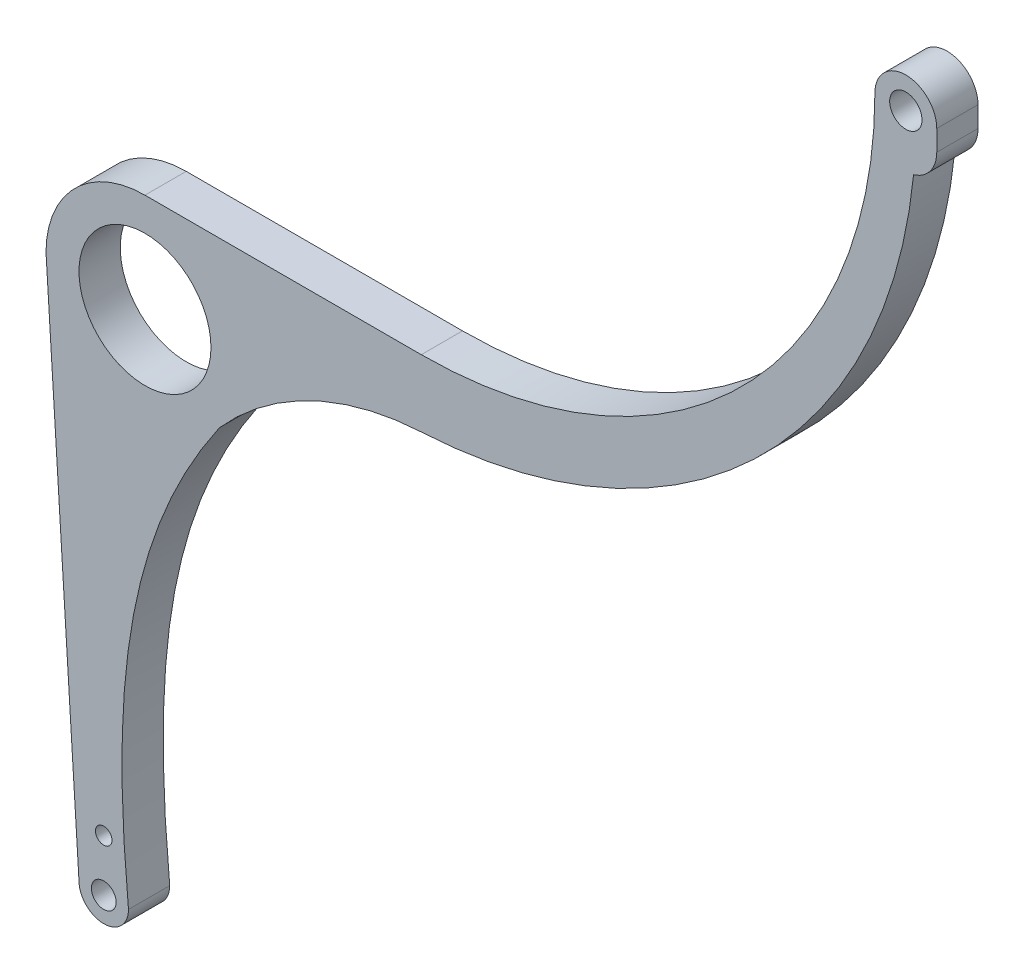
from build123d import *

# Parameters (mm, degrees)
SKETCH_1_R      = 3
SKETCH_1_R_2    = 16
SKETCH_1_R_3    = 3.91899873
SKETCH_1_R_4    = 2
EXTRUDE_1_DEPTH = 10


with BuildPart() as part:
    # 草图1 → 凸台-拉伸1 (new body)
    with BuildSketch(Plane.XY):
        with BuildLine():
            Line((-14, 128), (-6, 0))
            ThreePointArc((-6, 0), (0, -6), (6, 0))
            add(Edge.make_bspline(
                [(6, 0), (1.588652615, 45.680929706), (5.604102499, 79.643200211), (28.004797731, 112.13093391)],
                knots=[0, 0, 0, 0, 0.788155359, 0.788155359, 0.788155359, 0.788155359], degree=3))
            ThreePointArc((28.004797731, 112.13093391), (50.113637924, 128.900750568), (77, 135.767416406))
            ThreePointArc((77, 135.767416406), (157.787149523, 170.485384951), (196.379869136, 249.494896157))
            ThreePointArc((196.379869136, 249.494896157), (200.439238403, 252.311917913), (202, 257))
            Line((202, 257), (202, 262))
            ThreePointArc((202, 262), (194.5, 269.5), (187, 262))
            ThreePointArc((187, 262), (154.781745931, 184.218254069), (77, 152))
            Line((77, 152), (10, 152))
            ThreePointArc((10, 152), (-6.970562748, 144.970562748), (-14, 128))
        make_face()
        Circle(SKETCH_1_R, mode=Mode.SUBTRACT)
        with Locations((10, 128)):
            Circle(SKETCH_1_R_2, mode=Mode.SUBTRACT)
        with Locations((194.5, 262)):
            Circle(SKETCH_1_R_3, mode=Mode.SUBTRACT)
        with Locations((0, 12.5)):
            Circle(SKETCH_1_R_4, mode=Mode.SUBTRACT)
    extrude(amount=EXTRUDE_1_DEPTH)


solid = part.part
